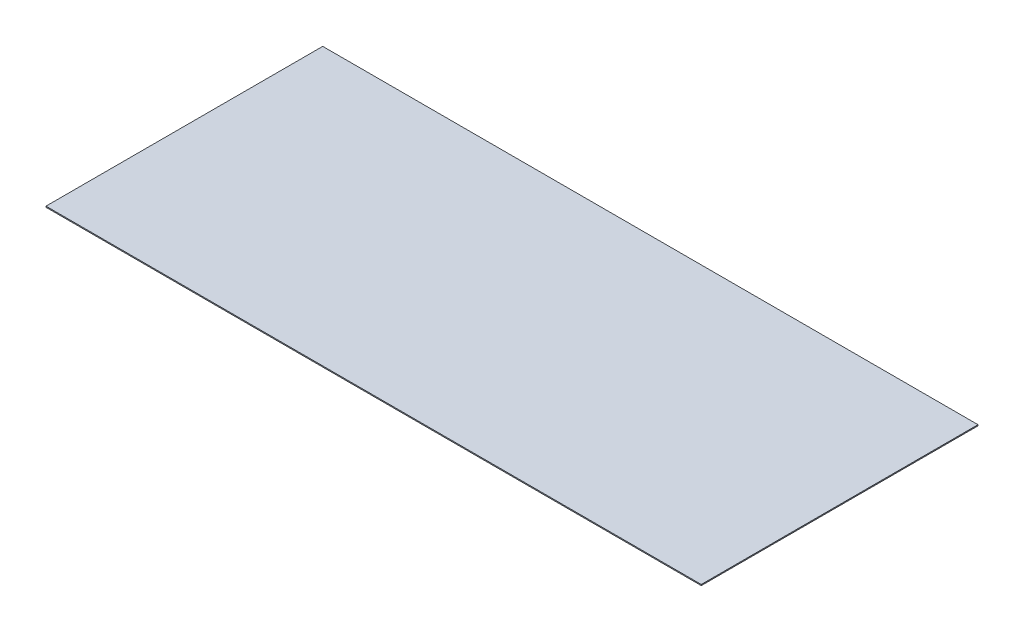
from build123d import *

# Parameters (mm, degrees)
SKETCH_1_W           = 5020
SKETCH_1_H           = 2120
BOSS_EXTRUDE_1_DEPTH = 8


with BuildPart() as part:
    # Sketch 1 → Boss-Extrude 1 (new body)
    with BuildSketch(Plane(origin=(0, 0, 0), x_dir=(1, 0, 0), z_dir=(0, 1, 0))):
        Rectangle(SKETCH_1_W, SKETCH_1_H)
    extrude(amount=BOSS_EXTRUDE_1_DEPTH)


solid = part.part
